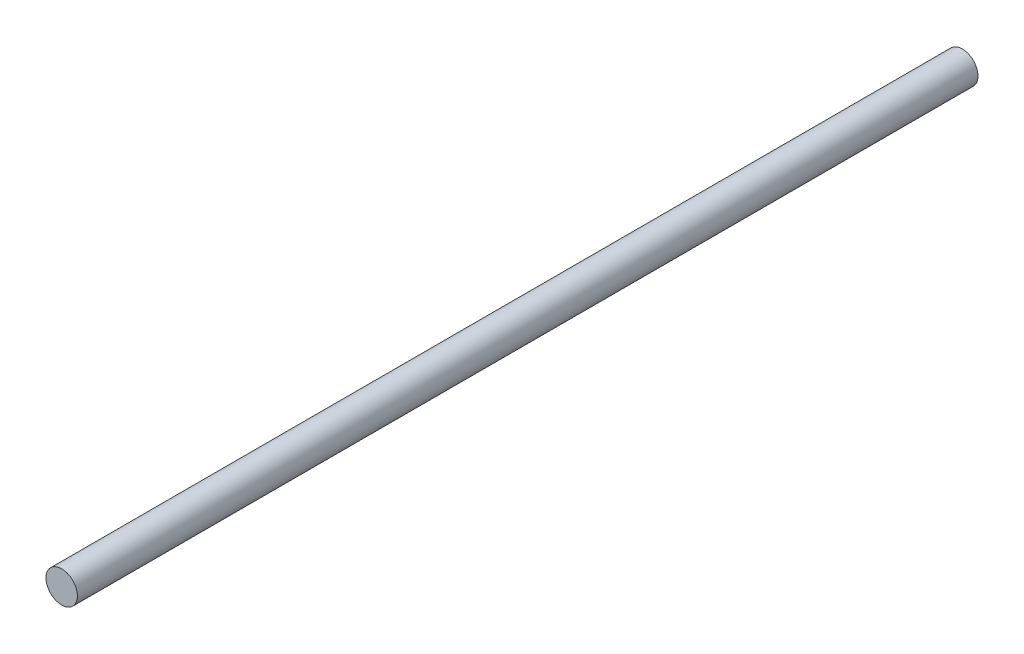
SolidWorks part; units mm, degrees
ref_plane "前视基准面" through (0, 0, 0) normal (0, 0, 1) x (1, 0, 0)
ref_plane "上视基准面" through (0, 0, 0) normal (0, 1, 0) x (1, 0, 0)
ref_plane "右视基准面" through (0, 0, 0) normal (1, 0, 0) x (0, 0, -1)
sketch "草图1" plane through (0, 0, 0) normal (0, 0, 1) x (1, 0, 0)
  circle A0 centre (0, 0) radius 7.5
  dimension "D1" = 15
extrude "凸台-拉伸1" add sketch "草图1" along normal blind 430
